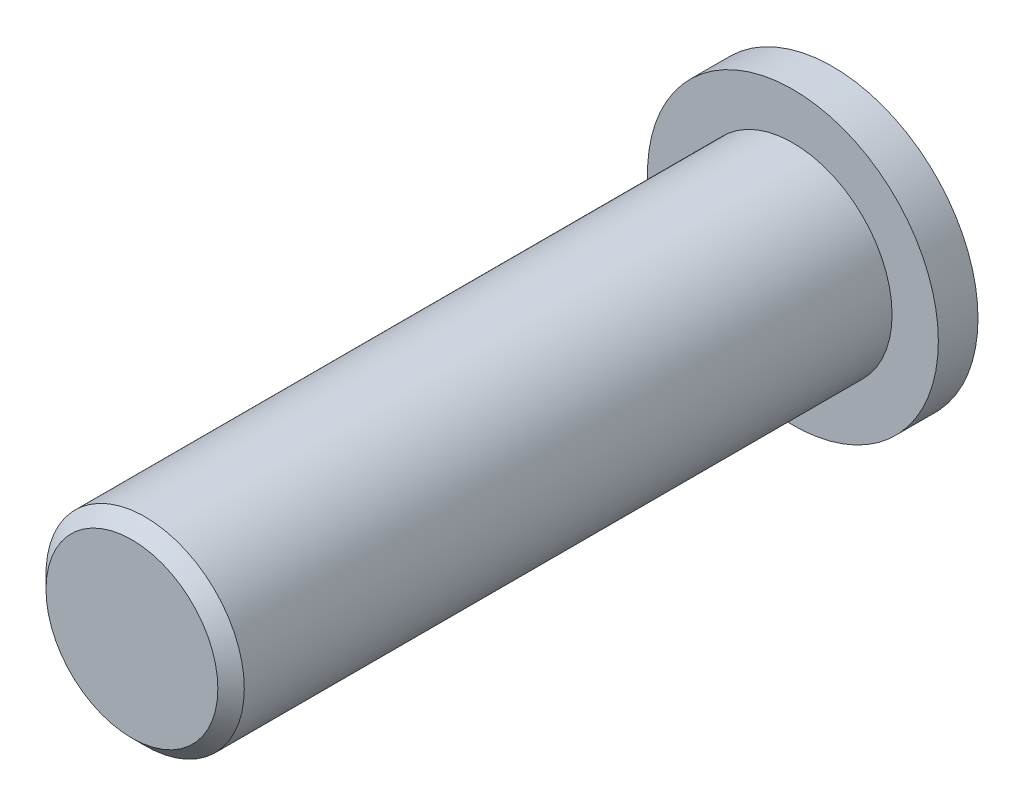
from build123d import *

# Parameters (mm, degrees)
SKETCH_1_R      = 11
EXTRUDE_1_DEPTH = 3
SKETCH_2_R      = 7.5
EXTRUDE_2_DEPTH = 50
CHAMFER_1_SIZE  = 1


with BuildPart() as part:
    # 草图1 → 凸台-拉伸1 (new body)
    with BuildSketch(Plane.XY):
        Circle(SKETCH_1_R)
    extrude(amount=EXTRUDE_1_DEPTH)

    # 草图2 → 凸台-拉伸2 (add)
    with BuildSketch(Plane.XY.offset(3)):
        Circle(SKETCH_2_R)
    extrude(amount=EXTRUDE_2_DEPTH)

    # 倒角1
    chamfer_1_edges = [part.edges().sort_by_distance(p)[0] for p in [
        (-7.5, 0, 53),
    ]]
    chamfer(chamfer_1_edges, length=CHAMFER_1_SIZE)


solid = part.part
